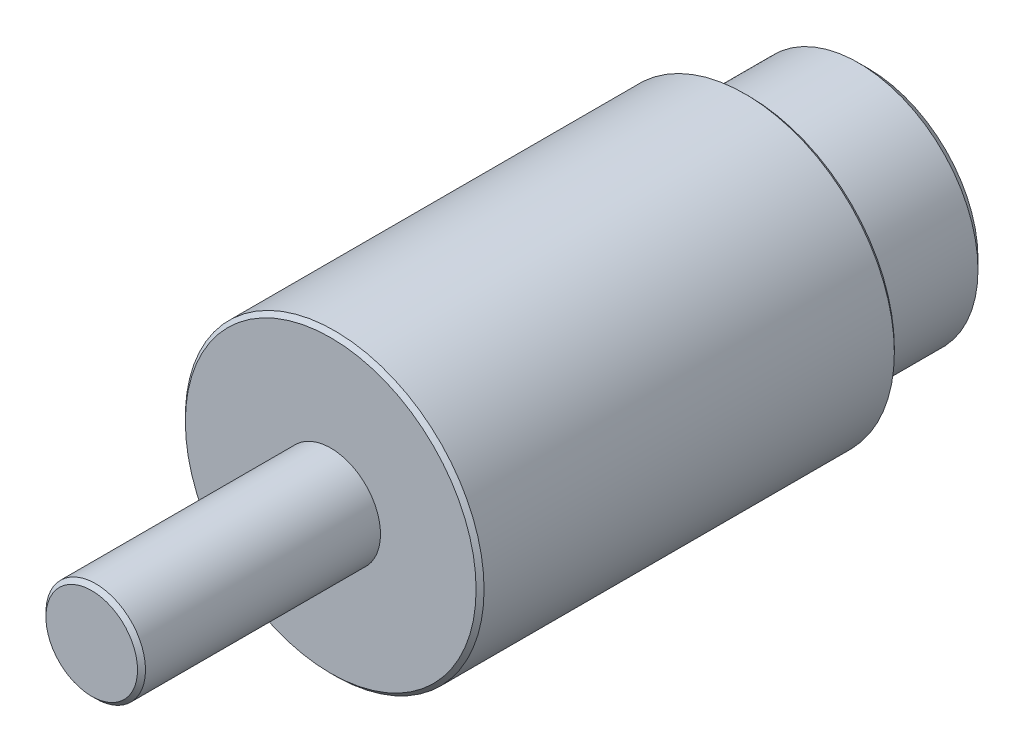
from build123d import *

# Parameters (mm, degrees)
SKETCH_1_R      = 6
EXTRUDE_1_DEPTH = 13.5
CHAMFER_1_SIZE  = 0.5
SKETCH_2_R      = 2.5
EXTRUDE_2_DEPTH = 12
CHAMFER_2_SIZE  = 0.2
SKETCH_3_R      = 7.5
EXTRUDE_3_DEPTH = 21
CHAMFER_3_SIZE  = 0.2


with BuildPart() as part:
    # 草图1 → 凸台-拉伸1 (new, symmetric)
    with BuildSketch(Plane.XY):
        Circle(SKETCH_1_R)
    extrude(amount=EXTRUDE_1_DEPTH, both=True)

    # 倒角1
    chamfer_1_edges = [part.edges().sort_by_distance(p)[0] for p in [
        (-6, 0, -13.5),
        (-6, 0, 13.5),
    ]]
    chamfer(chamfer_1_edges, length=CHAMFER_1_SIZE)

    # 草图2 → 凸台-拉伸2 (add)
    with BuildSketch(Plane.XY.offset(13.5)):
        Circle(SKETCH_2_R)
    extrude(amount=EXTRUDE_2_DEPTH)

    # 倒角2
    chamfer_2_edges = [part.edges().sort_by_distance(p)[0] for p in [
        (-2.5, 0, 25.5),
    ]]
    chamfer(chamfer_2_edges, length=CHAMFER_2_SIZE)

    # 草图3 → 凸台-拉伸3 (add)
    with BuildSketch(Plane.XY.offset(13.5)):
        Circle(SKETCH_3_R)
    extrude(amount=-EXTRUDE_3_DEPTH)

    # 倒角3
    chamfer_3_edges = [part.edges().sort_by_distance(p)[0] for p in [
        (-7.5, 0, 13.5),
        (-7.5, 0, -7.5),
    ]]
    chamfer(chamfer_3_edges, length=CHAMFER_3_SIZE)


solid = part.part
